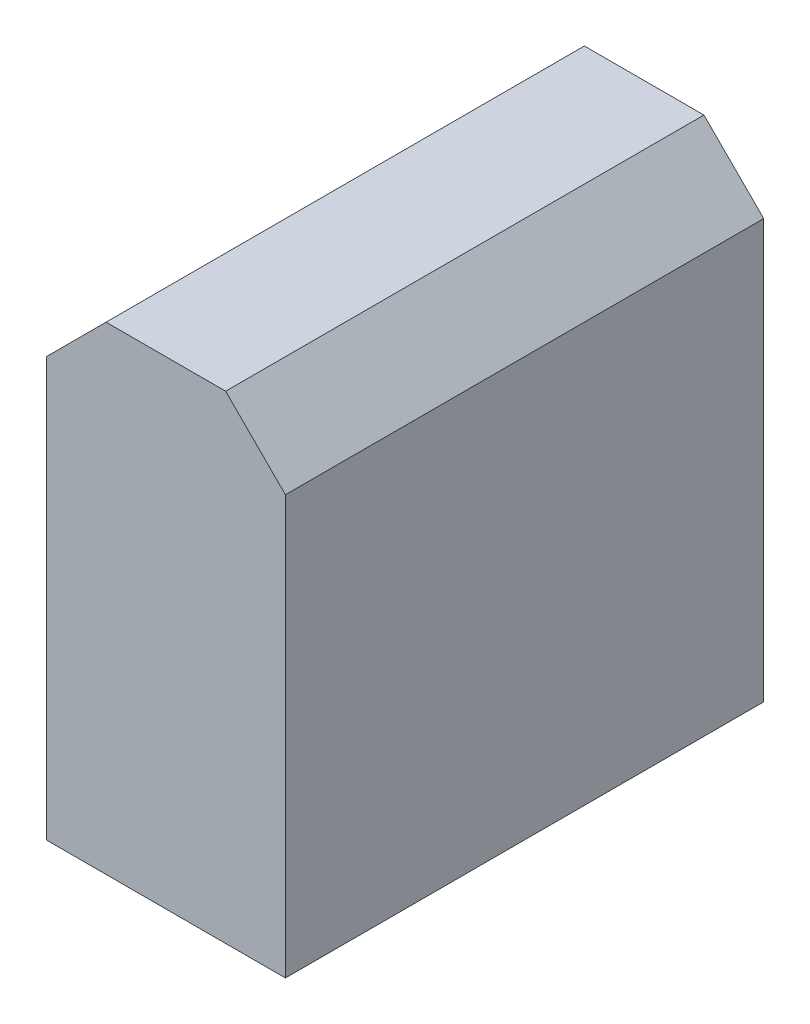
from build123d import *

# Parameters (mm, degrees)
SKETCH1_W           = 20
SKETCH1_H           = 40
BOSS_EXTRUDE1_DEPTH = 40
CHAMFER1_SIZE       = 5


with BuildPart() as part:
    # Sketch1 → Boss-Extrude1 (new body)
    with BuildSketch(Plane.XY):
        Rectangle(SKETCH1_W, SKETCH1_H)
    extrude(amount=BOSS_EXTRUDE1_DEPTH)

    # Chamfer1
    chamfer1_edges = [part.edges().sort_by_distance(p)[0] for p in [
        (-10, 20, 20),
        (10, 20, 20),
    ]]
    chamfer(chamfer1_edges, length=CHAMFER1_SIZE)


solid = part.part
